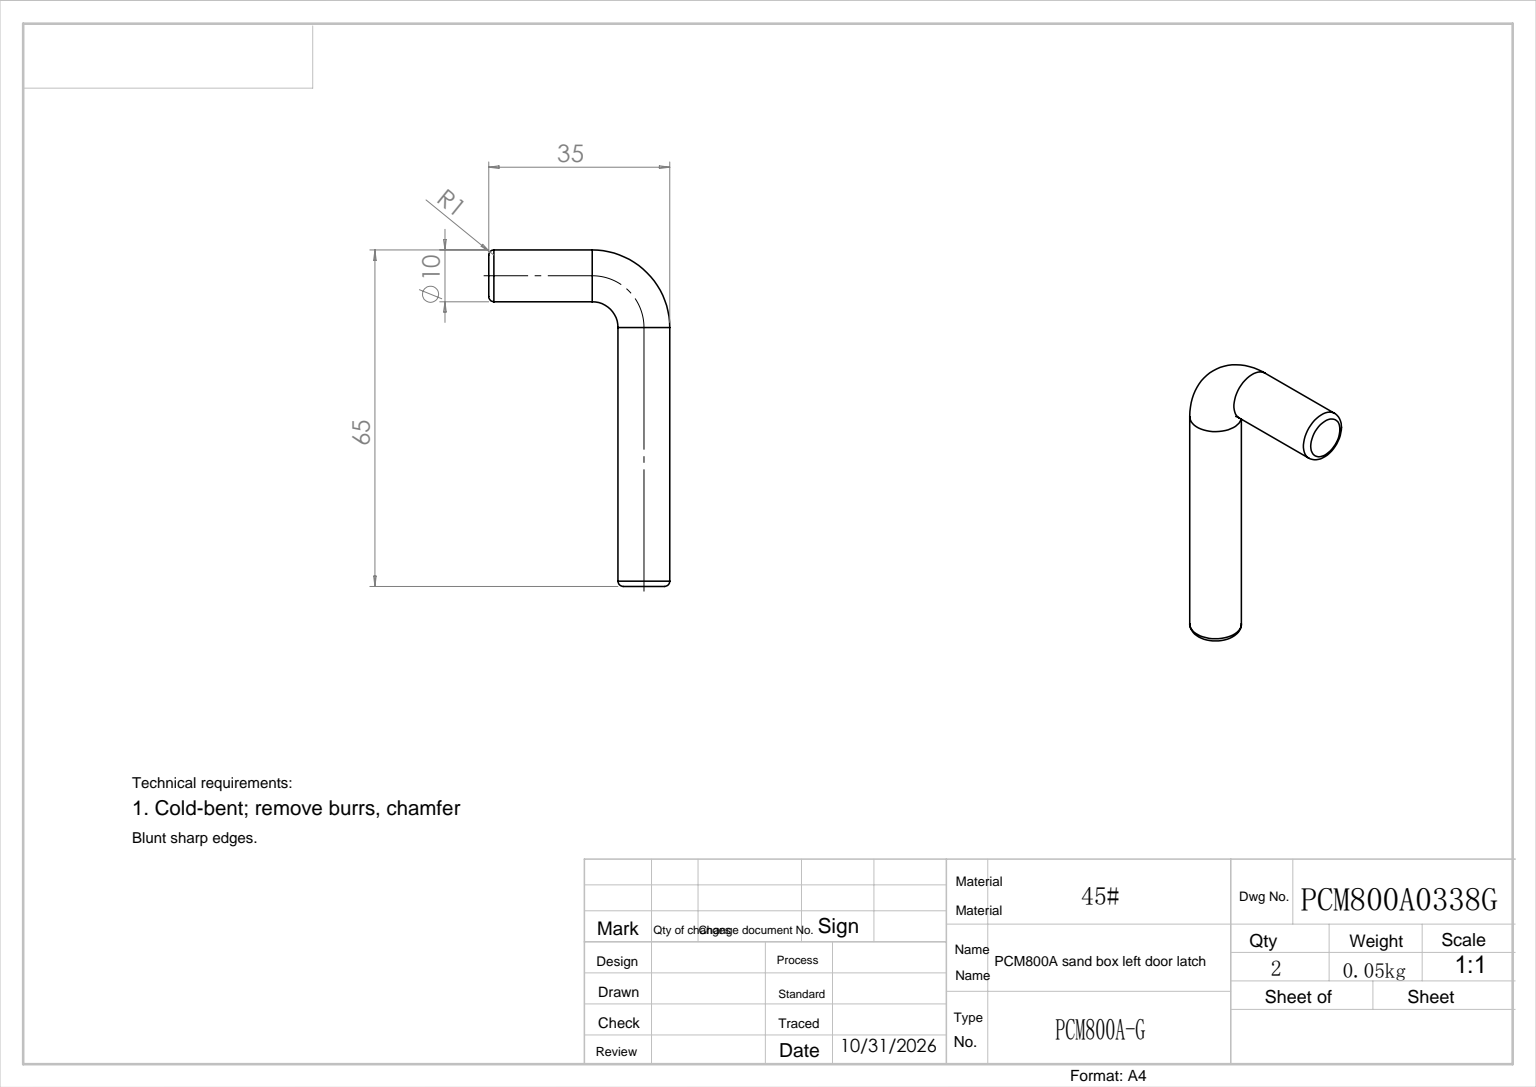
from build123d import *

# Parameters (mm, degrees)
SKETCH_2_R = 5
FILLET_1_R = 1


with BuildPart() as part:
    # 扫描1: sweep along a path in 草图1
    with BuildLine(Plane.XY) as sweep_1_path:
        Line((0, 0), (-20, 0))
        ThreePointArc((-20, 0), (-27.071067812, -2.928932188), (-30, -10))
        Line((-30, -10), (-30, -60))
    # 草图2 → 扫描1 (sweep)
    with BuildSketch(Plane(origin=(0, 0, 0), x_dir=(0, 0, -1), z_dir=(1, 0, 0))):
        Circle(SKETCH_2_R)
    sweep(path=sweep_1_path.line)

    # 圆角1
    fillet_1_edges = [part.edges().sort_by_distance(p)[0] for p in [
        (0, 0, 5),
        (-30, -60, 5),
    ]]
    fillet(fillet_1_edges, radius=FILLET_1_R)


solid = part.part
